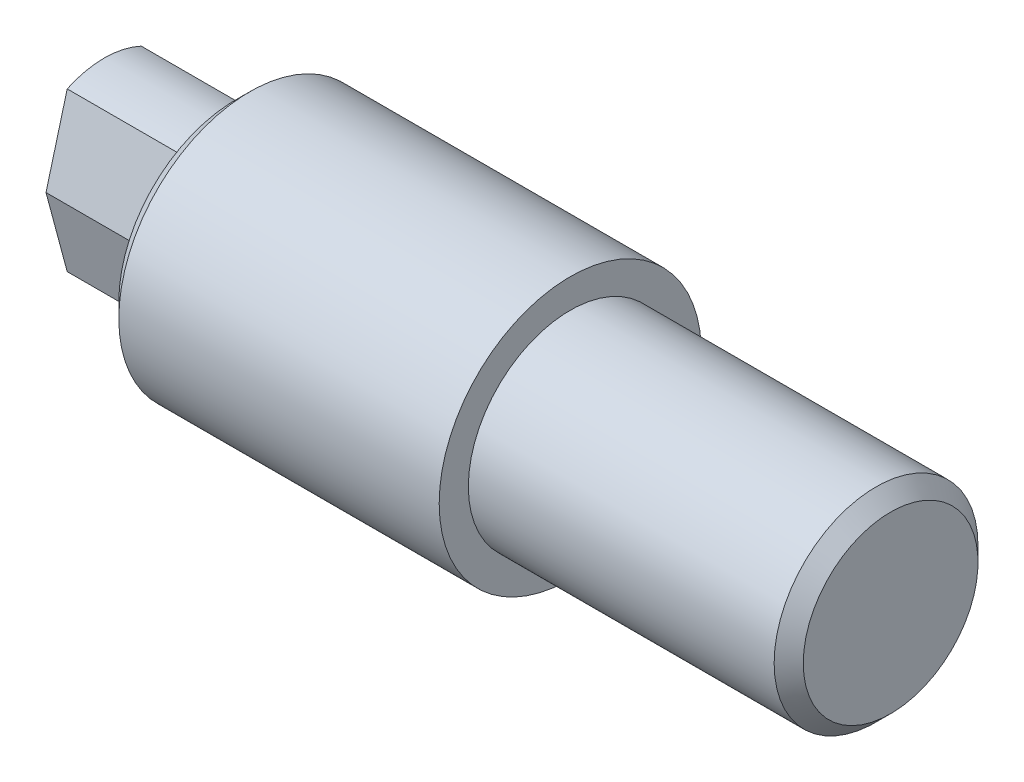
from build123d import *

# Parameters (mm, degrees)
CHAMFER1_SIZE       = 1
CHAMFER2_SIZE       = 1
BOSS_EXTRUDE1_DEPTH = 9


with BuildPart() as part:
    # Sketch1 → Revolve1 (revolve)
    with BuildSketch(Plane.XY, mode=Mode.PRIVATE) as revolve1_sk:
        Polygon((-21.47270101, 0), (-21.47270101, 9), (1.52729899, 9), (1.52729899, 7), (23.52729899, 7), (23.52729899, 0), align=None)
    revolve(revolve1_sk.sketch.rotate(Axis((-65.318854856, 0, 0), (1, 0, 0)), 90), axis=Axis((-65.318854856, 0, 0), (1, 0, 0)))

    # Chamfer1
    chamfer1_edges = [part.edges().sort_by_distance(p)[0] for p in [
        (23.52729899, 0, -7),
    ]]
    chamfer(chamfer1_edges, length=CHAMFER1_SIZE)

    # Chamfer2
    chamfer2_edges = [part.edges().sort_by_distance(p)[0] for p in [
        (-21.47270101, 0, -9),
    ]]
    chamfer(chamfer2_edges, length=CHAMFER2_SIZE)

    # Sketch3 → Boss-Extrude1 (add)
    with BuildSketch(Plane.ZY.offset(21.47270101)):
        with BuildLine():
            Line((4, 0), (2.543967169, 5.433988502))
            ThreePointArc((2.543967169, 5.433988502), (0, 6), (-2.543967169, 5.433988502))
            Line((-2.543967169, 5.433988502), (-4, 0))
            Line((-4, 0), (-2.543967169, -5.433988502))
            ThreePointArc((-2.543967169, -5.433988502), (0, -6), (2.543967169, -5.433988502))
            Line((2.543967169, -5.433988502), (4, 0))
        make_face()
    extrude(amount=BOSS_EXTRUDE1_DEPTH)


solid = part.part
